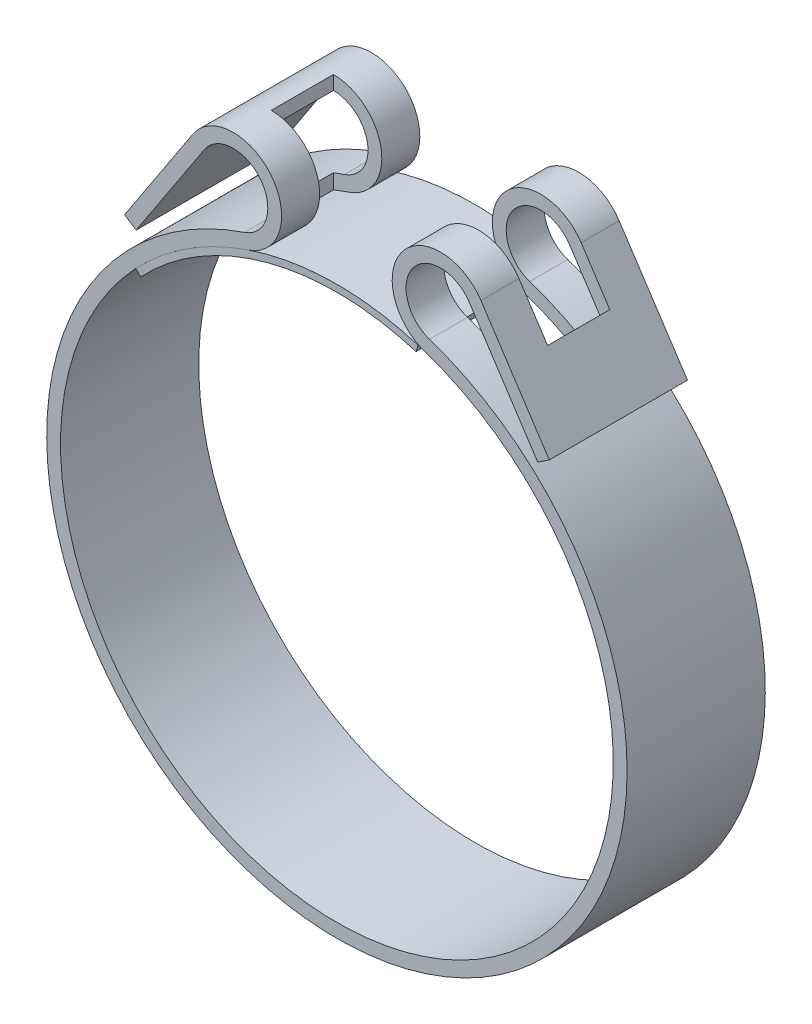
SolidWorks part; units mm, degrees
ref_plane "前视基准面" through (0, 0, 0) normal (0, 0, 1) x (1, 0, 0)
ref_plane "上视基准面" through (0, 0, 0) normal (0, 1, 0) x (1, 0, 0)
ref_plane "右视基准面" through (0, 0, 0) normal (1, 0, 0) x (0, 0, -1)
sketch "草图1" plane through (0, 0, 0) normal (0, 0, 1) x (1, 0, 0)
  line L0 (0, 0) -> (0, 52.2102) construction
  line L1 (19.1783, 47.2884) -> (29.0649, 32.2467)
  line L2 (-20.8496, 48.3869) -> (-30.7363, 33.3452)
  line L3 (-19.1783, 47.2884) -> (-29.0649, 32.2467)
  line L4 (20.8496, 48.3869) -> (30.7363, 33.3452)
  line L5 (-30.7363, 33.3452) -> (-29.0649, 32.2467)
  line L6 (29.0649, 32.2467) -> (30.7363, 33.3452)
  arc A0 (-13.4043, 39.8036) -> (13.4043, 39.8036) centre (0, 0) ccw
  arc A1 (-13.4043, 39.8036) -> (-19.1783, 47.2884) centre (-15, 44.5421) ccw
  arc A2 (13.4043, 39.8036) -> (19.1783, 47.2884) centre (15, 44.5421) cw
  arc A3 (-12.766, 37.9082) -> (-20.8496, 48.3869) centre (-15, 44.5421) ccw
  arc A4 (-12.766, 37.9082) -> (12.766, 37.9082) centre (0, 0) ccw
  arc A5 (12.766, 37.9082) -> (20.8496, 48.3869) centre (15, 44.5421) cw
  dimension "D1" = 84
  dimension "D4" = 10
  dimension "D5" = 2
  dimension "D2" = 15
  dimension "D3" = 18
extrude "凸台-拉伸1" add sketch "草图1" along normal blind 20
sketch "草图3" plane through (0, 0, 0) normal (0, 1, 0) x (1, 0, 0)
  line L1 (-15, -5.5) -> (5, -5.5)
  line L2 (-15, -5.5) -> (-15, -14.5)
  line L3 (-15, -14.5) -> (5, -14.5)
  line L4 (5, -5.5) -> (5, -14.5)
  line L5 (-15, -5.5) -> (5, -14.5) construction
  line L6 (-15, -14.5) -> (5, -5.5) construction
  point P0 (-5, -10)
  dimension "D1" = 10
  dimension "D2" = 9
  dimension "D3" = 20
  dimension "D4" = 5
extrude "切除-拉伸1" cut sketch "草图3" along normal blind 60
ref_plane "基准面1" through (0, 51.5421, 0) normal (0, 1, 0) x (1, 0, 0)
sketch "草图4" plane through (0, 51.5421, 0) normal (0, 1, 0) x (1, 0, 0)
  line L1 (0, -5.5) -> (25, -5.5)
  line L2 (0, -5.5) -> (0, -14.5)
  line L3 (0, -14.5) -> (25, -14.5)
  line L4 (25, -5.5) -> (25, -14.5)
  dimension "D1" = 9
  dimension "D2" = 5.5
  dimension "D3" = 25
  dimension "D4" = 0
extrude "切除-拉伸2" cut sketch "草图4" against normal blind 60
sketch "草图5" plane through (0, 0, 0) normal (0, 0, 1) x (1, 0, 0)
  line L0 (-28.3899, 26.7397) -> (-29.1179, 27.4253)
  line L1 (11.4564, 37.2794) -> (11.7501, 38.2353)
  arc A0 (11.7501, 38.2353) -> (-29.1179, 27.4253) centre (0, 0) ccw
  arc A1 (11.4564, 37.2794) -> (-28.3899, 26.7397) centre (0, 0) ccw
  circle A2 centre (0, 0) radius 39 construction
  circle A3 centre (0, 0) radius 40 construction
  arc A4 (-12.766, 37.9082) -> (12.766, 37.9082) centre (0, 0) ccw construction
  dimension "D1" = 1
extrude "凸台-拉伸2" add sketch "草图5" along normal blind 20 separate body
